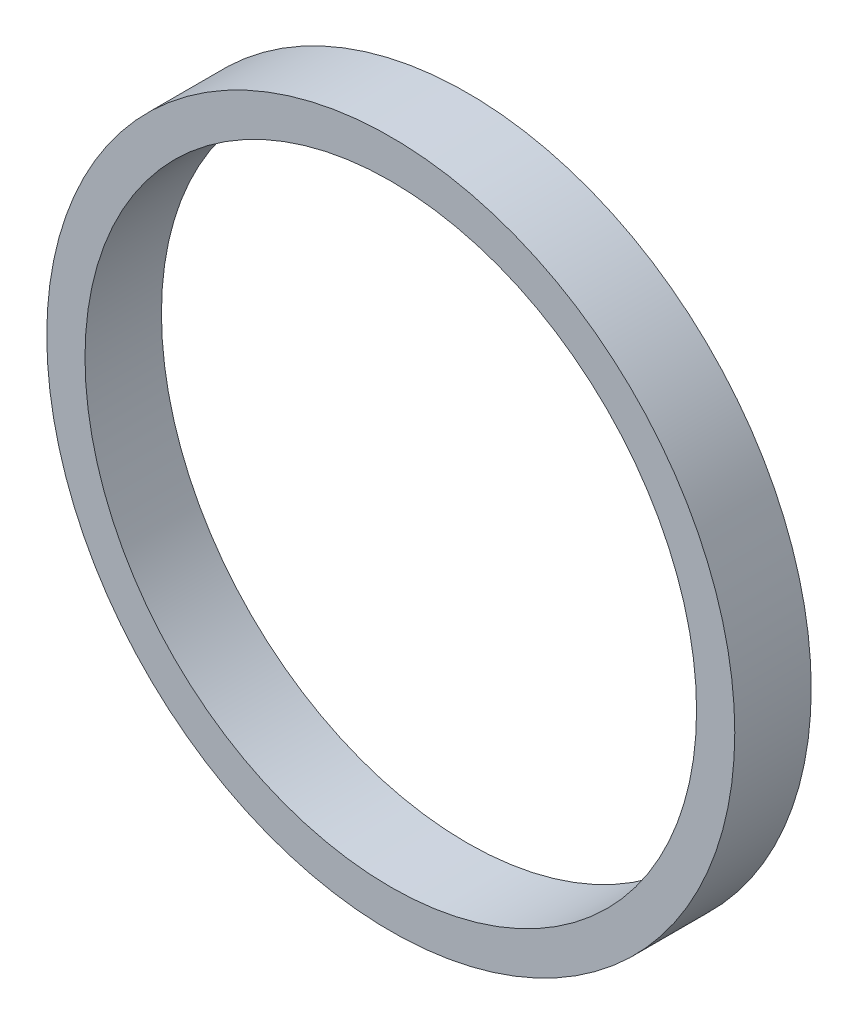
SolidWorks part; units mm, degrees
ref_plane "Front Plane" through (0, 0, 0) normal (0, 0, 1) x (1, 0, 0)
ref_plane "Top Plane" through (0, 0, 0) normal (0, 1, 0) x (1, 0, 0)
ref_plane "Right Plane" through (0, 0, 0) normal (1, 0, 0) x (0, 0, -1)
sketch "Sketch1" plane through (0, 0, 0) normal (0, 0, 1) x (1, 0, 0)
  circle A0 centre (0, 0) radius 4.5
  circle A1 centre (0, 0) radius 4
  dimension "D1" = 8
  dimension "D2" = 9
extrude "Boss-Extrude1" add sketch "Sketch1" along normal blind 1
